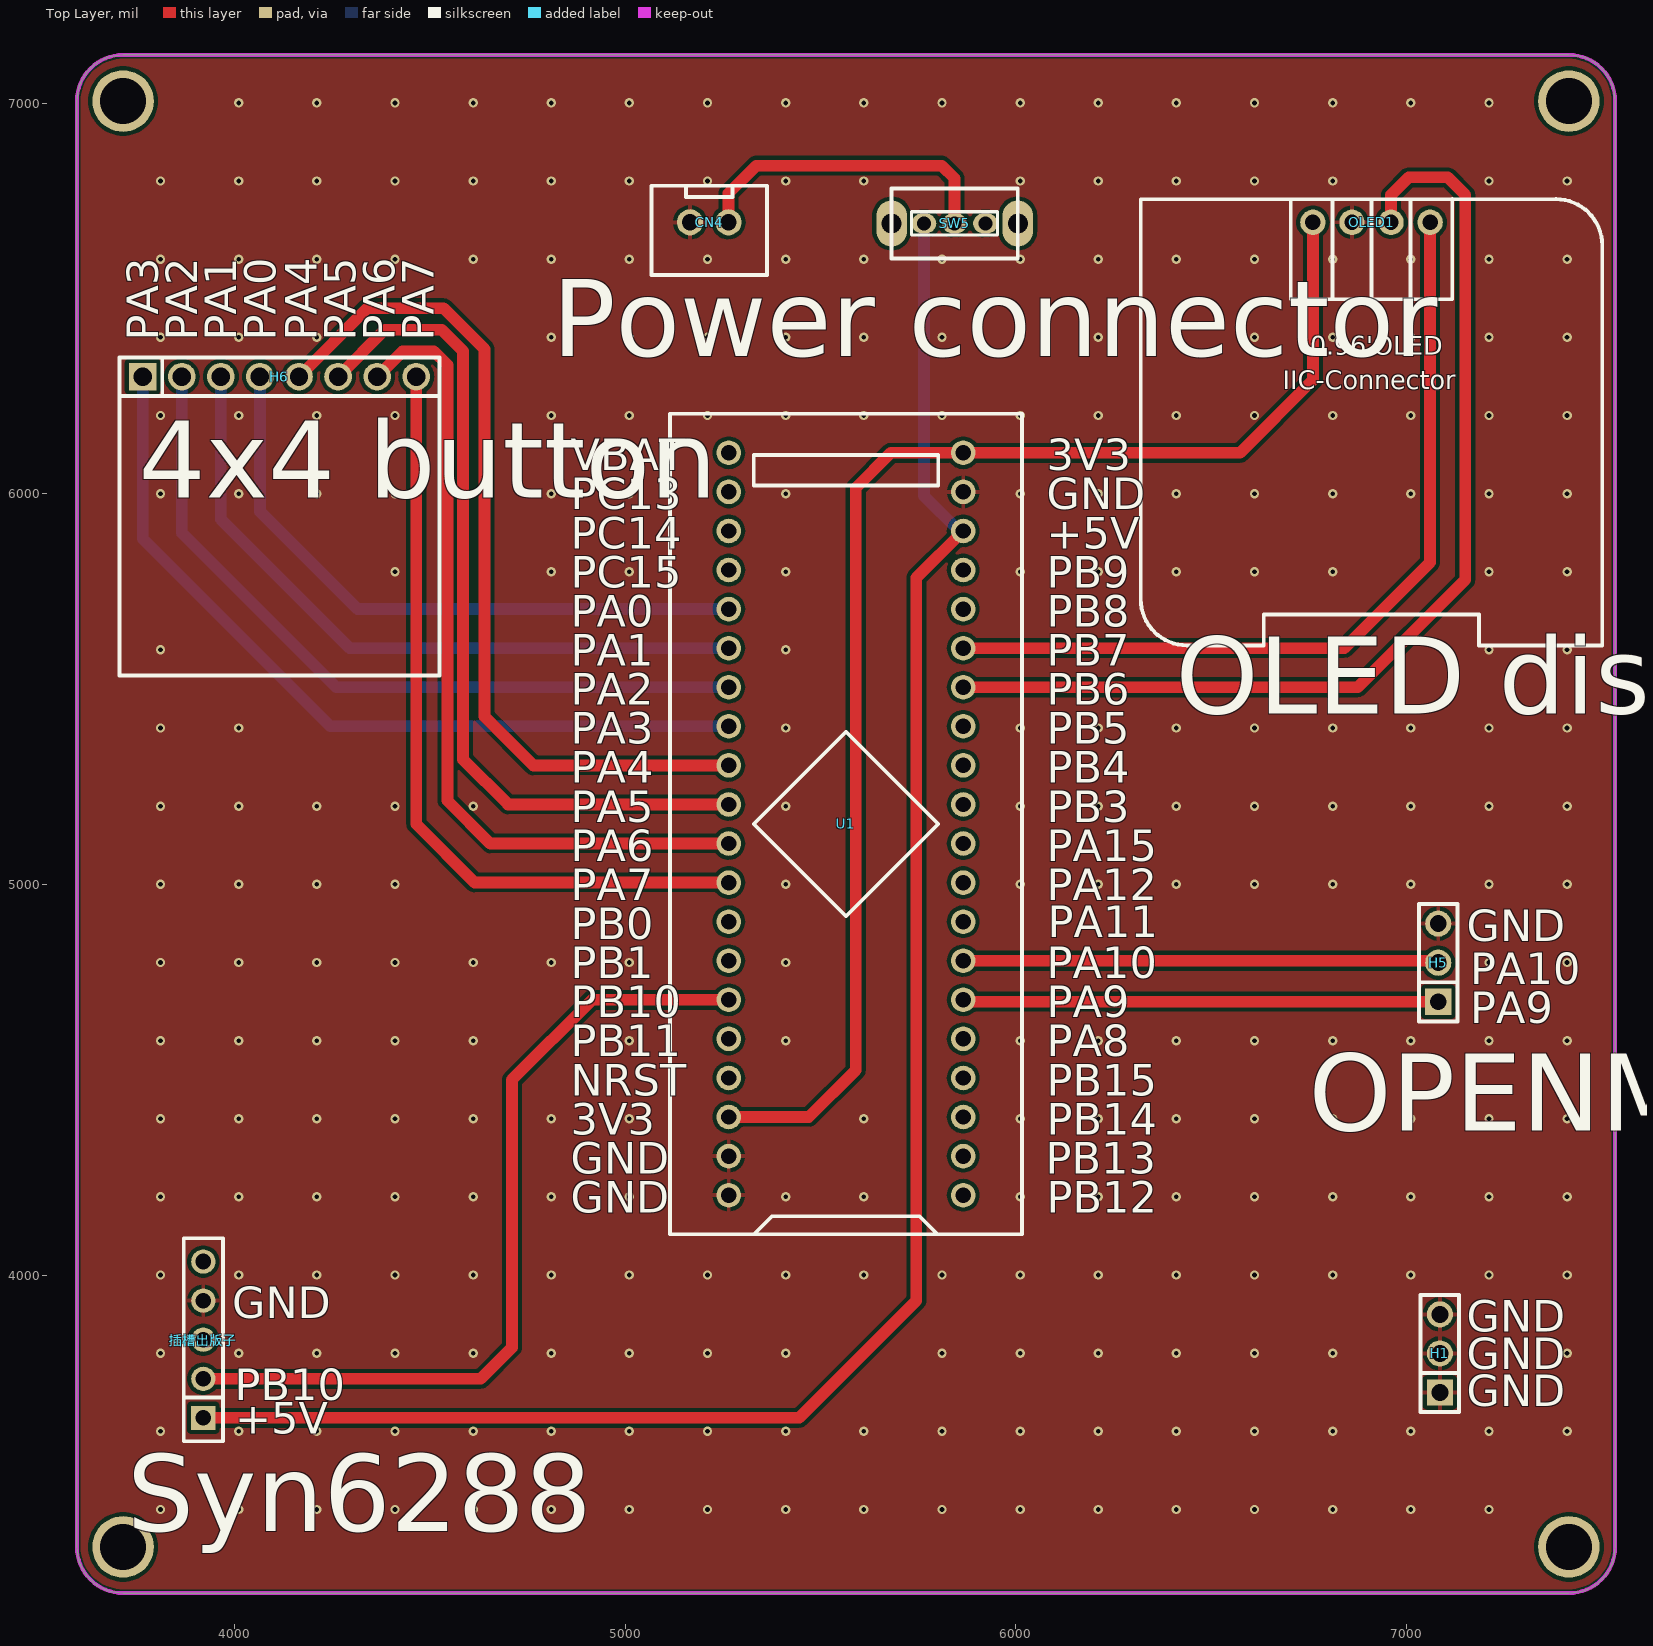
[diagram p0: Top Layer view]
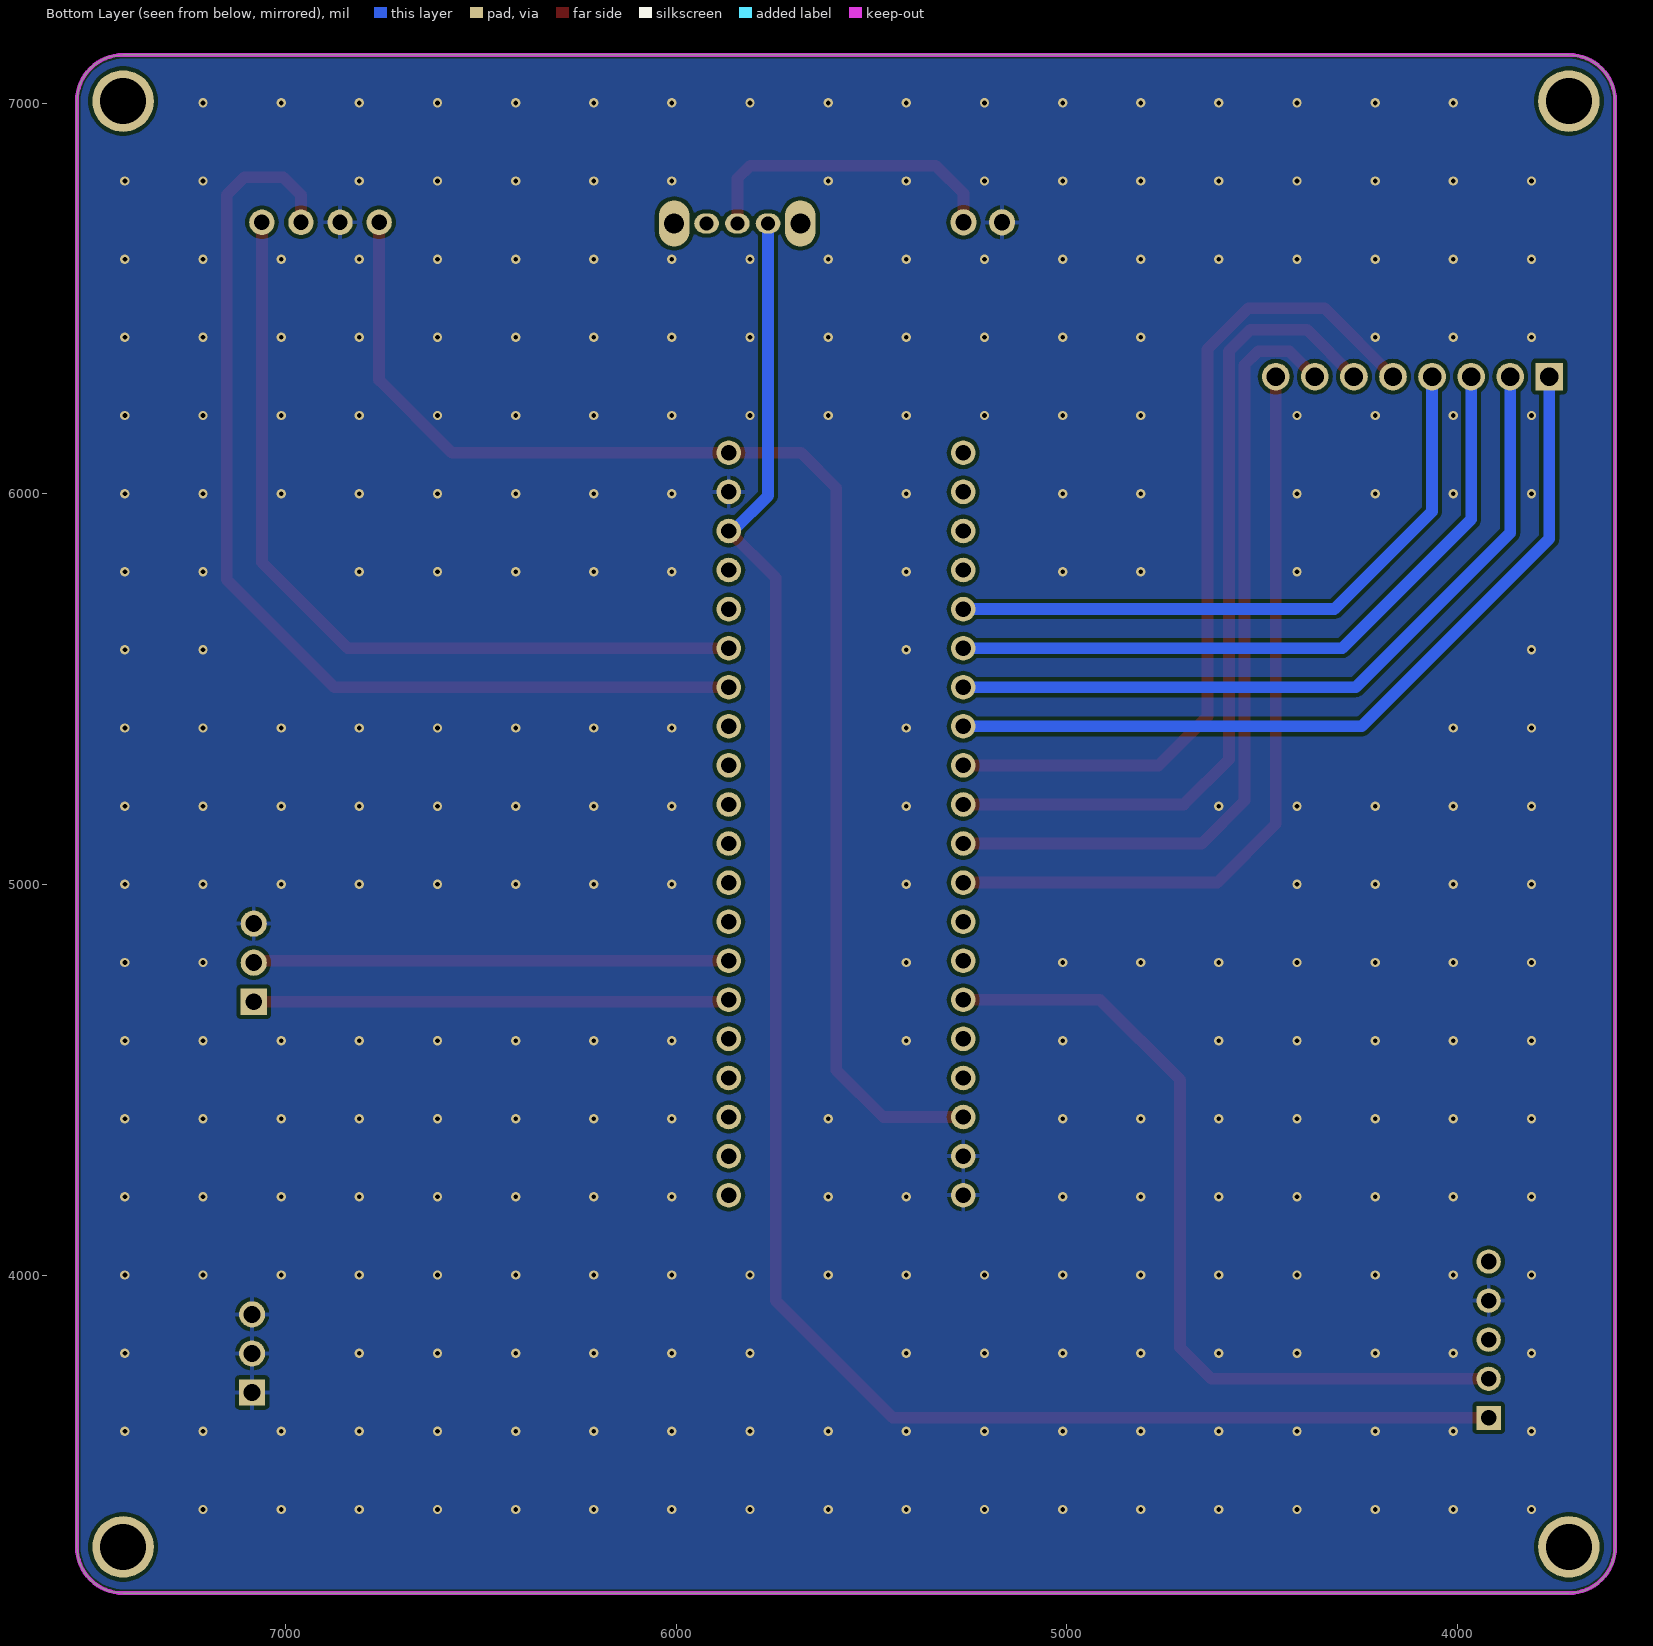
[diagram p1: Bottom Layer view, seen from below]
# Altium PCB MISC51713.pcbdoc
Units mil, origin at the board's own origin, x right, y up, seen from the top; angles counter-clockwise.
Board outline 3937.01 x 3937.01 mil, 2 copper layers (Top Layer, Bottom Layer), stack 62.206 mil thick; 8 components, 38 nets, 74 pads, 286 vias.

## Layer stack, top to bottom
Top Solder Mask Layer: solder mask 0.394, Dk 3.3
Top Layer: signal copper 1.379
Dielectric1: surface 59.449, FR4, Dk 4.5
Bottom Layer: signal copper 1.378
Bottom Solder Mask Layer: solder mask 0.394, Dk 3.3

## Board outline
3714.61,7123.5 ccw(c3714.61,7005.39) 3596.5,7005.39 3596.5,3304.61 ccw(c3714.61,3304.61) 3714.61,3186.5 7415.39,3186.5 ccw(c7415.39,3304.61) 7533.5,3304.61 7533.5,7005.39 ccw(c7415.39,7005.39) 7415.39,7123.5 3714.61,7123.5

## Design rules (kind name [scope] priority, off if disabled: settings)
BoardOutlineClearance copperThickness2oz_1 [All] p2 off: genericclearance=7.99 ignorepadtopadclearanceinfootprint=FALSE except(0: Arc-SplitContinuation Track-SplitContinuation SMDPad-SplitContinuation THPad-SplitContinuation Via-SplitContinuation Fill-SplitContinuation Region-SplitContinuation Poly-SplitContinuation Text-SplitContinuation Hole-SplitContinuation; 5.98: Arc-CutoutEdge Track-CutoutEdge SMDPad-CutoutEdge THPad-CutoutEdge Via-CutoutEdge Text-CutoutEdge; 6.9: Hole-OutlineEdge Hole-CutoutEdge; 10: Poly-OutlineEdge Poly-CutoutEdge; 11.81: Arc-OutlineEdge Track-OutlineEdge SMDPad-OutlineEdge THPad-OutlineEdge Via-OutlineEdge Fill-OutlineEdge Region-OutlineEdge Text-OutlineEdge Fill-CutoutEdge Region-CutoutEdge)
BoardOutlineClearance Plane_innerPlane_1 [All] p4 off: genericclearance=4.02 ignorepadtopadclearanceinfootprint=FALSE except(0: Arc-SplitContinuation Track-SplitContinuation SMDPad-SplitContinuation THPad-SplitContinuation Via-SplitContinuation Fill-SplitContinuation Region-SplitContinuation Poly-SplitContinuation Text-SplitContinuation Hole-SplitContinuation; 5.98: Arc-CutoutEdge Track-CutoutEdge SMDPad-CutoutEdge THPad-CutoutEdge Via-CutoutEdge Text-CutoutEdge; 6.9: Hole-OutlineEdge Hole-CutoutEdge; 10: Poly-OutlineEdge Poly-CutoutEdge; 11.81: Arc-OutlineEdge Track-OutlineEdge SMDPad-OutlineEdge THPad-OutlineEdge Via-OutlineEdge Fill-OutlineEdge Region-OutlineEdge Text-OutlineEdge Fill-CutoutEdge Region-CutoutEdge)
BoardOutlineClearance Copper_copperRegion_1 [All] p6 off: genericclearance=4.02 ignorepadtopadclearanceinfootprint=FALSE except(0: Arc-SplitContinuation Track-SplitContinuation SMDPad-SplitContinuation THPad-SplitContinuation Via-SplitContinuation Fill-SplitContinuation Region-SplitContinuation Poly-SplitContinuation Text-SplitContinuation Hole-SplitContinuation; 5.98: Arc-CutoutEdge Track-CutoutEdge SMDPad-CutoutEdge THPad-CutoutEdge Via-CutoutEdge Text-CutoutEdge; 6.9: Hole-OutlineEdge Hole-CutoutEdge; 10: Poly-OutlineEdge Poly-CutoutEdge; 11.81: Arc-OutlineEdge Track-OutlineEdge SMDPad-OutlineEdge THPad-OutlineEdge Via-OutlineEdge Fill-OutlineEdge Region-OutlineEdge Text-OutlineEdge Fill-CutoutEdge Region-CutoutEdge)
BoardOutlineClearance Copper_copperRegion_copperThickness1oz_1 [All] p8 off: genericclearance=4.02 ignorepadtopadclearanceinfootprint=FALSE except(0: Arc-SplitContinuation Track-SplitContinuation SMDPad-SplitContinuation THPad-SplitContinuation Via-SplitContinuation Fill-SplitContinuation Region-SplitContinuation Poly-SplitContinuation Text-SplitContinuation Hole-SplitContinuation; 5.98: Arc-CutoutEdge Track-CutoutEdge SMDPad-CutoutEdge THPad-CutoutEdge Via-CutoutEdge Text-CutoutEdge; 6.9: Hole-OutlineEdge Hole-CutoutEdge; 10: Poly-OutlineEdge Poly-CutoutEdge; 11.81: Arc-OutlineEdge Track-OutlineEdge SMDPad-OutlineEdge THPad-OutlineEdge Via-OutlineEdge Fill-OutlineEdge Region-OutlineEdge Text-OutlineEdge Fill-CutoutEdge Region-CutoutEdge)
BoardOutlineClearance Copper_copperRegion_Copper_copperRegion_1 [All] p10 off: genericclearance=4.02 ignorepadtopadclearanceinfootprint=FALSE except(0: Arc-SplitContinuation Track-SplitContinuation SMDPad-SplitContinuation THPad-SplitContinuation Via-SplitContinuation Fill-SplitContinuation Region-SplitContinuation Poly-SplitContinuation Text-SplitContinuation Hole-SplitContinuation; 5.98: Arc-CutoutEdge Track-CutoutEdge SMDPad-CutoutEdge THPad-CutoutEdge Via-CutoutEdge Text-CutoutEdge; 6.9: Hole-OutlineEdge Hole-CutoutEdge; 10: Poly-OutlineEdge Poly-CutoutEdge; 11.81: Arc-OutlineEdge Track-OutlineEdge SMDPad-OutlineEdge THPad-OutlineEdge Via-OutlineEdge Fill-OutlineEdge Region-OutlineEdge Text-OutlineEdge Fill-CutoutEdge Region-CutoutEdge)
BoardOutlineClearance copperThickness1oz_1 [All] p12: genericclearance=4.02 ignorepadtopadclearanceinfootprint=FALSE except(0: Arc-SplitContinuation Track-SplitContinuation SMDPad-SplitContinuation THPad-SplitContinuation Via-SplitContinuation Fill-SplitContinuation Region-SplitContinuation Poly-SplitContinuation Text-SplitContinuation Hole-SplitContinuation; 5.98: Arc-CutoutEdge Track-CutoutEdge SMDPad-CutoutEdge THPad-CutoutEdge Via-CutoutEdge Text-CutoutEdge; 6.9: Hole-OutlineEdge Hole-CutoutEdge; 10: Poly-OutlineEdge Poly-CutoutEdge; 11.81: Arc-OutlineEdge Track-OutlineEdge SMDPad-OutlineEdge THPad-OutlineEdge Via-OutlineEdge Fill-OutlineEdge Region-OutlineEdge Text-OutlineEdge Fill-CutoutEdge Region-CutoutEdge)
Clearance copperThickness2oz [All] p1 off: gap=7.99 ignorepadtopadclearanceinfootprint=FALSE except(5.98: SMDPad-Track SMDPad-SMDPad THPad-Track SMDPad-THPad THPad-THPad Track-Via SMDPad-Via THPad-Via Via-Via Fill-SMDPad Region-SMDPad Fill-THPad Region-THPad Fill-Via Region-Via Fill-Fill Fill-Region Region-Region Arc-Track Arc-SMDPad Arc-THPad Arc-Via Fill-Arc Region-Arc Arc-Arc Text-Track SMDPad-Text Text-THPad Text-Via Fill-Text Region-Text Arc-Text Text-Text; 6.9: Hole-Track Hole-SMDPad Hole-THPad Hole-Via Fill-Hole Region-Hole Hole-Arc Hole-Text; 10: Poly-Track Poly-SMDPad Poly-THPad Poly-Via Poly-Fill Poly-Region Poly-Poly Poly-Arc Poly-Text Poly-Hole; 11.81: Fill-Track Region-Track)
Clearance Plane_innerPlane [All] p3 off: gap=4.02 ignorepadtopadclearanceinfootprint=FALSE except(5.98: SMDPad-Track SMDPad-SMDPad THPad-Track SMDPad-THPad THPad-THPad Track-Via SMDPad-Via THPad-Via Via-Via Fill-SMDPad Region-SMDPad Fill-THPad Region-THPad Fill-Via Region-Via Fill-Fill Fill-Region Region-Region Arc-Track Arc-SMDPad Arc-THPad Arc-Via Fill-Arc Region-Arc Arc-Arc Text-Track SMDPad-Text Text-THPad Text-Via Fill-Text Region-Text Arc-Text Text-Text; 6.9: Hole-Track Hole-SMDPad Hole-THPad Hole-Via Fill-Hole Region-Hole Hole-Arc Hole-Text; 10: Poly-Track Poly-SMDPad Poly-THPad Poly-Via Poly-Fill Poly-Region Poly-Poly Poly-Arc Poly-Text Poly-Hole; 11.81: Fill-Track Region-Track)
Clearance Copper_copperRegion [All] p5 off: gap=4.02 ignorepadtopadclearanceinfootprint=FALSE except(5.98: SMDPad-Track SMDPad-SMDPad THPad-Track SMDPad-THPad THPad-THPad Track-Via SMDPad-Via THPad-Via Via-Via Fill-SMDPad Region-SMDPad Fill-THPad Region-THPad Fill-Via Region-Via Fill-Fill Fill-Region Region-Region Arc-Track Arc-SMDPad Arc-THPad Arc-Via Fill-Arc Region-Arc Arc-Arc Text-Track SMDPad-Text Text-THPad Text-Via Fill-Text Region-Text Arc-Text Text-Text; 6.9: Hole-Track Hole-SMDPad Hole-THPad Hole-Via Fill-Hole Region-Hole Hole-Arc Hole-Text; 10: Poly-Track Poly-SMDPad Poly-THPad Poly-Via Poly-Fill Poly-Region Poly-Poly Poly-Arc Poly-Text Poly-Hole; 11.81: Fill-Track Region-Track)
Clearance Copper_copperRegion_copperThickness1oz [All] p7 off: gap=4.02 ignorepadtopadclearanceinfootprint=FALSE except(5.98: SMDPad-Track SMDPad-SMDPad THPad-Track SMDPad-THPad THPad-THPad Track-Via SMDPad-Via THPad-Via Via-Via Fill-SMDPad Region-SMDPad Fill-THPad Region-THPad Fill-Via Region-Via Fill-Fill Fill-Region Region-Region Arc-Track Arc-SMDPad Arc-THPad Arc-Via Fill-Arc Region-Arc Arc-Arc Text-Track SMDPad-Text Text-THPad Text-Via Fill-Text Region-Text Arc-Text Text-Text; 6.9: Hole-Track Hole-SMDPad Hole-THPad Hole-Via Fill-Hole Region-Hole Hole-Arc Hole-Text; 10: Poly-Track Poly-SMDPad Poly-THPad Poly-Via Poly-Fill Poly-Region Poly-Poly Poly-Arc Poly-Text Poly-Hole; 11.81: Fill-Track Region-Track)
Clearance Copper_copperRegion_Copper_copperRegion [All] p9 off: gap=4.02 ignorepadtopadclearanceinfootprint=FALSE except(5.98: SMDPad-Track SMDPad-SMDPad THPad-Track SMDPad-THPad THPad-THPad Track-Via SMDPad-Via THPad-Via Via-Via Fill-SMDPad Region-SMDPad Fill-THPad Region-THPad Fill-Via Region-Via Fill-Fill Fill-Region Region-Region Arc-Track Arc-SMDPad Arc-THPad Arc-Via Fill-Arc Region-Arc Arc-Arc Text-Track SMDPad-Text Text-THPad Text-Via Fill-Text Region-Text Arc-Text Text-Text; 6.9: Hole-Track Hole-SMDPad Hole-THPad Hole-Via Fill-Hole Region-Hole Hole-Arc Hole-Text; 10: Poly-Track Poly-SMDPad Poly-THPad Poly-Via Poly-Fill Poly-Region Poly-Poly Poly-Arc Poly-Text Poly-Hole; 11.81: Fill-Track Region-Track)
Clearance copperThickness1oz [All] p11: gap=4.02 ignorepadtopadclearanceinfootprint=FALSE except(5.98: SMDPad-Track SMDPad-SMDPad THPad-Track SMDPad-THPad THPad-THPad Track-Via SMDPad-Via THPad-Via Via-Via Fill-SMDPad Region-SMDPad Fill-THPad Region-THPad Fill-Via Region-Via Fill-Fill Fill-Region Region-Region Arc-Track Arc-SMDPad Arc-THPad Arc-Via Fill-Arc Region-Arc Arc-Arc Text-Track SMDPad-Text Text-THPad Text-Via Fill-Text Region-Text Arc-Text Text-Text; 6.9: Hole-Track Hole-SMDPad Hole-THPad Hole-Via Fill-Hole Region-Hole Hole-Arc Hole-Text; 10: Poly-Track Poly-SMDPad Poly-THPad Poly-Via Poly-Fill Poly-Region Poly-Poly Poly-Arc Poly-Text Poly-Hole; 11.81: Fill-Track Region-Track)
DiffPairsRouting differentialPair [All] p1: maxlimit=6 minlimit=6 mostfreqgap=6 toplayer_minwidth=5 toplayer_prefwidth=10 toplayer_maxwidth=100 toplayer_mingap=6 toplayer_prefgap=6 toplayer_maxgap=6 bottomlayer_minwidth=5 bottomlayer_prefwidth=10 bottomlayer_maxwidth=100 bottomlayer_mingap=6 bottomlayer_prefgap=6 bottomlayer_maxgap=6 maxuncoupledlength=10
HoleToHoleClearance otherClearance [All] p1: gap=11.81 allowstackedmicrovias=TRUE
Length netLength [All] p1: minlimit=0 maxlimit=0
PasteMaskExpansion pasteMaskExpansion [All] p1: expansion=0
PlaneConnect innerPlane [All] p1: planeconnectstyle=Relief reliefexpansion=20 reliefentries=4 reliefconductorwidth=10 reliefairgap=10
PolygonConnect copperRegion_copperThickness1oz [All] p1 off: connectstyle=Relief reliefconductorwidth=10 reliefentries=4 polygonreliefangle="90 Angle" airgapwidth=10 via.connectstyle=Relief via.reliefconductorwidth=10 via.reliefentries=4 via.polygonreliefangle="90 Angle" via.airgapwidth=10
PolygonConnect copperRegion_Copper_copperRegion [All] p2 off: connectstyle=Relief reliefconductorwidth=10 reliefentries=4 polygonreliefangle="90 Angle" airgapwidth=10 via.connectstyle=Relief via.reliefconductorwidth=10 via.reliefentries=4 via.polygonreliefangle="90 Angle" via.airgapwidth=10
PolygonConnect copperRegion [All] p3: connectstyle=Relief reliefconductorwidth=10 reliefentries=4 polygonreliefangle="90 Angle" airgapwidth=10 via.connectstyle=Relief via.reliefconductorwidth=10 via.reliefentries=4 via.polygonreliefangle="90 Angle" via.airgapwidth=10
RoutingVias viaSize [All] p1: holewidth=12.01 width=24.02 viastyle="Through Hole" minholewidth=11.81 minwidth=19.68 maxholewidth=248.03 maxwidth=393.7
SolderMaskExpansion solderMaskExpansion [IsVia] p1: expansion=-1000 istentingtop=TRUE
SolderMaskExpansion solderMaskExpansion [All] p2: expansion=2 istentingtop=FALSE
Width copperThickness2oz_2 [All] p1 off: maxlimit=100 minlimit=8 preferedwidth=10
Width copperThickness1oz_2 [All] p2: maxlimit=100 minlimit=5 preferedwidth=10

## Components (designator, comment, footprint, x,y, rotation, side; value= is the part's Value field where it differs from the comment)
CN4 "XH2.54*2P_Through-hole" CONN-TH_2P-P2.50-XH2.54-2P 5215,6695 r0 top
H1 "" HDR-TH_3P-P2.54-V-M 7085,3800 r90 top
H5 "" HDR-TH_3P-P2.54-V-M 7080.79,4800 r90 top
H6 "" HDR-TH_8P-P2.54-V-F-1 4115,6300 r0 top
OLED1 "" 0.96OLED_4P 6910,6695 r0 top
SW5 "" 拨动开关 5837.9,6692.05 r0 top
U1 "STM32F103C8T6-Card" CONN-TH_L53.3-W22.9_STM32F103C8T6-CARD 5565,5155 r90 top
插槽出版子 "" HDR-TH_5P-P2.54-V-F 3920,3835 r90 top

## Footprints (in the part's own frame and the unit in brackets; to place one, negate y for a bottom-side part, rotate by r counter-clockwise, add the part's x,y. Pads: shape width x height; smd on the part's side, far side on the other; paste and mask are expansions set on the pad)
0.96OLED_4P [mm]
  round 1.65 hole 1 copper offset 0,0: 1(-3.81,-0.001) 2(-1.27,0.002) 3(1.27,0.002) 4(3.81,0.002)
  silkscreen extent -15,-27.5 15,1.5
CONN-TH_2P-P2.50-XH2.54-2P [mm]
  round 1.7 hole 1.05 paste+0 mask+0.05: 1(1.25,0) 2(-1.25,0)
  silkscreen extent -3.75,-3.42 3.75,2.37
CONN-TH_L53.3-W22.9_STM32F103C8T6-CARD [mm]
  round 1.6 hole 1: 1(-24.13,-7.62) 2(-21.59,-7.62) 3(-19.05,-7.62) 4(-16.51,-7.62) 5(-13.97,-7.62) 6(-11.43,-7.62) 7(-8.89,-7.62) 8(-6.35,-7.62) 9(-3.81,-7.62) 10(-1.27,-7.62) 11(1.27,-7.62) 12(3.81,-7.62) 13(6.35,-7.62) 14(8.89,-7.62) 15(11.43,-7.62) 16(13.97,-7.62) 17(16.51,-7.62) 18(19.05,-7.62) 19(21.59,-7.62) 20(24.13,-7.62) 21(24.13,7.62) 22(21.59,7.62) 23(19.05,7.62) 24(16.51,7.62) 25(13.97,7.62) 26(11.43,7.62) 27(8.89,7.62) 28(6.35,7.62) 29(3.81,7.62) 30(1.27,7.62) 31(-1.27,7.62) 32(-3.81,7.62) 33(-6.35,7.62) 34(-8.89,7.62) 35(-11.43,7.62) 36(-13.97,7.62) 37(-16.51,7.62) 38(-19.05,7.62) 39(-21.59,7.62) 40(-24.13,7.62)
  silkscreen extent -26.67,-11.43 26.67,11.43
HDR-TH_3P-P2.54-V-M [mm]
  rect 1.7x1.7 hole 1.1: 1(-2.54,0)
  round 1.7 hole 1.1: 2(0,0) 3(2.54,0)
  silkscreen extent -3.81,-1.25 3.81,1.25
HDR-TH_5P-P2.54-V-F [mil]
  rect 62x62 hole 40.16: 1(-200,0)
  round 62 hole 40.16: 2(-100,0) 3(0,0) 4(100,0) 5(200,0)
  silkscreen extent -260,-50 260,50
HDR-TH_8P-P2.54-V-F-1 [mm]
  rect 1.8x1.8 hole 1.2: 1(-8.89,0)
  round 1.8 hole 1.2: 2(-6.35,0) 3(-3.81,0) 4(-1.27,0) 5(1.27,0) 6(3.81,0) 7(6.35,0) 8(8.89,0)
  silkscreen extent -10.41,-1.25 10.41,1.25
拨动开关 [mil]
  oval 63x51.2 hole 35.4 paste+0 mask+2: 1(-73.4,0) 2(5,0) 3(84,0)
  oval 78.7x118.1 hole 51.2 paste+0 mask+2: 4(166.7,0) 5(-156.1,0)
  silkscreen extent -156,-90 167,90

## Free pads (board coordinates)
  round 157.48 hole 118.11: 1(3714.61,7005.39) 1(3714.61,3304.61) 1(7415.39,7005.39) 1(7415.39,3304.61)

## Via types
v1: diameter 24.02, hole 12, Top Layer to Bottom Layer, 286 vias

## Nets (pads, with @x,y where several pads share a name; then routed paths per layer and width w, separated by ;. In a path a pad name is that pad's centre, name@x,y a point inside that pad or via, vN(x,y) a via of type N, cw(c..) or ccw(c..) an arc to the next point about the centre after c; other vN are vias at no path point)
$1N17118: CN4.1 SW5.2 | length 810.9
  Top Layer w30: CN4.1 5264.22,6769.22 5335,6840 5810,6840 5842.9,6807.1 SW5.2
+5V: SW5.1 U1.18 插槽出版子.1 | length 4803.5
  Top Layer w30: 插槽出版子.1 5445,3635 5745,3935 5745,5785 U1.18
  Bottom Layer w30: SW5.1 5764.5,5995.5 5855,5905 U1.18
GND: CN4.2 H1.1 H1.2 H1.3 H5.3 OLED1.2 U1.19 U1.39 U1.40 插槽出版子.4
  other v1: 3810.6,3400.6 4010.6,3400.6 4210.6,3400.6 4410.6,3400.6 4610.6,3400.6 4810.6,3400.6 5010.6,3400.6 5210.6,3400.6 5410.6,3400.6 5610.6,3400.6 5810.6,3400.6 6010.6,3400.6 6210.6,3400.6 6410.6,3400.6 6610.6,3400.6 6810.6,3400.6 7010.6,3400.6 7210.6,3400.6 3810.6,3600.6 4010.6,3600.6 4210.6,3600.6 4410.6,3600.6 4610.6,3600.6 4810.6,3600.6 5010.6,3600.6 5210.6,3600.6 5410.6,3600.6 5610.6,3600.6 5810.6,3600.6 6010.6,3600.6 6210.6,3600.6 6410.6,3600.6 6610.6,3600.6 6810.6,3600.6 7010.6,3600.6 7210.6,3600.6 7410.6,3600.6 3810.6,3800.6 4010.6,3800.6 4210.6,3800.6 4410.6,3800.6 4610.6,3800.6 4810.6,3800.6 5010.6,3800.6 5210.6,3800.6 5410.6,3800.6 5810.6,3800.6 6010.6,3800.6 6210.6,3800.6 6410.6,3800.6 6610.6,3800.6 6810.6,3800.6 7410.6,3800.6 3810.6,4000.6 4010.6,4000.6 4210.6,4000.6 4410.6,4000.6 4610.6,4000.6 4810.6,4000.6 5010.6,4000.6 5210.6,4000.6 5410.6,4000.6 5610.6,4000.6 5810.6,4000.6 6010.6,4000.6 6210.6,4000.6 6410.6,4000.6 6610.6,4000.6 6810.6,4000.6 7010.6,4000.6 7210.6,4000.6 7410.6,4000.6 3810.6,4200.6 4010.6,4200.6 4210.6,4200.6 4410.6,4200.6 4610.6,4200.6 4810.6,4200.6 5010.6,4200.6 5410.6,4200.6 5610.6,4200.6 6010.6,4200.6 6210.6,4200.6 6410.6,4200.6 6610.6,4200.6 6810.6,4200.6 7010.6,4200.6 7210.6,4200.6 7410.6,4200.6 3810.6,4400.6 4010.6,4400.6 4210.6,4400.6 4410.6,4400.6 4610.6,4400.6 4810.6,4400.6 5010.6,4400.6 5610.6,4400.6 6010.6,4400.6 6210.6,4400.6 6410.6,4400.6 6610.6,4400.6 6810.6,4400.6 7010.6,4400.6 7210.6,4400.6 7410.6,4400.6 3810.6,4600.6 4010.6,4600.6 4210.6,4600.6 4410.6,4600.6 4610.6,4600.6 5010.6,4600.6 5410.6,4600.6 6010.6,4600.6 6210.6,4600.6 6410.6,4600.6 6610.6,4600.6 6810.6,4600.6 7010.6,4600.6 7210.6,4600.6 7410.6,4600.6 3810.6,4800.6 4010.6,4800.6 4210.6,4800.6 4410.6,4800.6 4610.6,4800.6 4810.6,4800.6 5010.6,4800.6 5410.6,4800.6 7210.6,4800.6 7410.6,4800.6 3810.6,5000.6 4010.6,5000.6 4210.6,5000.6 4410.6,5000.6 5410.6,5000.6 6010.6,5000.6 6210.6,5000.6 6410.6,5000.6 6610.6,5000.6 6810.6,5000.6 7010.6,5000.6 7210.6,5000.6 7410.6,5000.6 3810.6,5200.6 4010.6,5200.6 4210.6,5200.6 4410.6,5200.6 4610.6,5200.6 5410.6,5200.6 6010.6,5200.6 6210.6,5200.6 6410.6,5200.6 6610.6,5200.6 6810.6,5200.6 7010.6,5200.6 7210.6,5200.6 7410.6,5200.6 3810.6,5400.6 4010.6,5400.6 5410.6,5400.6 6010.6,5400.6 6210.6,5400.6 6410.6,5400.6 6610.6,5400.6 6810.6,5400.6 7010.6,5400.6 7210.6,5400.6 7410.6,5400.6 3810.6,5600.6 5410.6,5600.6 7210.6,5600.6 7410.6,5600.6 4410.6,5800.6 4810.6,5800.6 5010.6,5800.6 5410.6,5800.6 6010.6,5800.6 6210.6,5800.6 6410.6,5800.6 6610.6,5800.6 6810.6,5800.6 7210.6,5800.6 7410.6,5800.6 3810.6,6000.6 4010.6,6000.6 4210.6,6000.6 4410.6,6000.6 4810.6,6000.6 5010.6,6000.6 5410.6,6000.6 6010.6,6000.6 6210.6,6000.6 6410.6,6000.6 6610.6,6000.6 6810.6,6000.6 7010.6,6000.6 7210.6,6000.6 7410.6,6000.6 3810.6,6200.6 4010.6,6200.6 4210.6,6200.6 4410.6,6200.6 4810.6,6200.6 5010.6,6200.6 5210.6,6200.6 5410.6,6200.6 5610.6,6200.6 5810.6,6200.6 6010.6,6200.6 6210.6,6200.6 6410.6,6200.6 6610.6,6200.6 6810.6,6200.6 7010.6,6200.6 7210.6,6200.6 7410.6,6200.6 3810.6,6400.6 4010.6,6400.6 4210.6,6400.6 4810.6,6400.6 5010.6,6400.6 5210.6,6400.6 5410.6,6400.6 5610.6,6400.6 5810.6,6400.6 6010.6,6400.6 6210.6,6400.6 6410.6,6400.6 6610.6,6400.6 6810.6,6400.6 7010.6,6400.6 7210.6,6400.6 7410.6,6400.6 3810.6,6600.6 4010.6,6600.6 4210.6,6600.6 4410.6,6600.6 4610.6,6600.6 4810.6,6600.6 5010.6,6600.6 5210.6,6600.6 5410.6,6600.6 5610.6,6600.6 5810.6,6600.6 6010.6,6600.6 6210.6,6600.6 6410.6,6600.6 6610.6,6600.6 6810.6,6600.6 7010.6,6600.6 7210.6,6600.6 7410.6,6600.6 3810.6,6800.6 4010.6,6800.6 4210.6,6800.6 4410.6,6800.6 4610.6,6800.6 4810.6,6800.6 5010.6,6800.6 5210.6,6800.6 5410.6,6800.6 5610.6,6800.6 6010.6,6800.6 6210.6,6800.6 6410.6,6800.6 6610.6,6800.6 6810.6,6800.6 7210.6,6800.6 7410.6,6800.6 4010.6,7000.6 4210.6,7000.6 4410.6,7000.6 4610.6,7000.6 4810.6,7000.6 5010.6,7000.6 5210.6,7000.6 5410.6,7000.6 5610.6,7000.6 5810.6,7000.6 6010.6,7000.6 6210.6,7000.6 6410.6,7000.6 6610.6,7000.6 6810.6,7000.6 7010.6,7000.6 7210.6,7000.6
NRST: U1.37
PA0: H6.4 U1.25 | length 1648.6
  Bottom Layer w30: H6.4 4065,5955 4315,5705 U1.25
PA1: H6.3 U1.26 | length 1801.7
  Bottom Layer w30: H6.3 3965,5935 4295,5605 U1.26
PA2: H6.2 U1.27 | length 1963.6
  Bottom Layer w30: H6.2 3865,5900 4260,5505 U1.27
PA3: H6.1 U1.28 | length 2113.8
  Bottom Layer w30: H6.1 3765,5885 4245,5405 U1.28
PA4: H6.5 U1.29 | length 2207.8
  Top Layer w30: H6.5 4340,6475 4535,6475 4640,6370 4640,5430 4765,5305 U1.29
PA5: H6.6 U1.30 | length 2165.1
  Top Layer w30: H6.6 4385,6420 4530,6420 4585,6365 4585,5320 4700,5205 U1.30
PA6: H6.7 U1.31 | length 2102
  Top Layer w30: H6.7 4430,6365 4510,6365 4545,6330 4545,5215 4655,5105 U1.31
PA7: H6.8 U1.32 | length 2007.1
  Top Layer w30: H6.8 4465,5155 4615,5005 U1.32
PA8: U1.5
PA9: H5.1 U1.6 | length 1217.9
  Top Layer w30: U1.6 5870,4700 H5.1
PA10: H5.2 U1.7 | length 1217.9
  Top Layer w30: U1.7 7075.79,4805 H5.2
PA11: U1.8
PA12: U1.9
PA15: U1.10
PB0: U1.33
PB1: U1.34
PB3: U1.11
PB4: U1.12
PB5: U1.13
PB6: OLED1.3 U1.14 | length 2681.1
  Top Layer w30: U1.14 6875,5505 7150,5780 7150,6765 7105,6810 7005,6810 6960,6765 OLED1.3@6960,6695.05
PB7: OLED1.4 U1.15 | length 2156.2
  Top Layer w30: U1.15 6840,5605 7060,5825 OLED1.4@7060,6695.05
PB8: U1.16
PB9: U1.17
PB10: U1.35 插槽出版子.2 | length 2148.1
  Top Layer w30: 插槽出版子.2 4630,3735 4710,3815 4710,4500 4915,4705 U1.35
PB11: U1.36
PB12: U1.1
PB13: U1.2
PB14: U1.3
PB15: U1.4
PC13: U1.22
PC14: U1.23
PC15: U1.24
VBAT: U1.21
VCC: OLED1.1 U1.20 U1.38 | length 3552.7
  Top Layer w30: U1.38 5470,4405 5590,4525 5590,6015 5680,6105 U1.20 6573.61,6105 6760,6291.4 OLED1.1
pads on no net: SW5.3 SW5.4 SW5.5 插槽出版子.3 插槽出版子.5

## Polygon pours and split planes (outlines as drawn)
GND on Bottom Layer (solid, remove dead copper, pour order 2): 3525,7245 3525,3080 7700,3080 7700,7245
GND on Top Layer (solid, remove dead copper, pour order 2): 3000,7415 3000,3000 7930,3000 7930,7415

## Keep-outs
Board Outline Layer:
  the board outline again, w10

## Silkscreen, mask and mechanical layers (free items; w line width, h text height)
Top Silkscreen Layer:
  lines w10: 3705.16,5535 3705.16,6349.21 4525,6349.21 4525,5535 3705.16,5535
  text "PA3" at 3805,6391.55 h80 r90
  text "PA2" at 3905,6391.55 h80 r90
  text "PA1" at 4005,6391.55 h80 r90
  text "PA0" at 4105,6391.55 h80 r90
  text "PA4" at 4210,6391.55 h80 r90
  text "PA5" at 4310,6391.55 h80 r90
  text "PA6" at 4410,6391.55 h80 r90
  text "PA7" at 4510,6391.55 h80 r90
  text "Power connector" at 4812.87,6351.57 h196.85
  text "VBAT" at 4860.95,6060 h80
  text "3V3" at 6079.16,6060 h80
  text "4x4 button" at 3755,5990 h196.85
  text "PC13" at 4860.95,5960 h80
  text "GND" at 6079.16,5960 h80
  text "PC14" at 4860.95,5860 h80
  text "+5V" at 6079.16,5860 h80
  text "PC15" at 4860.95,5760 h80
  text "PB9" at 6079.16,5760 h80
  text "PA0" at 4860.95,5660 h80
  text "PB8" at 6079.16,5660 h80
  text "PA1" at 4860.95,5560 h80
  text "PB7" at 6079.16,5560 h80
  text "PA2" at 4860.95,5460 h80
  text "PB6" at 6079.16,5460 h80
  text "OLED display" at 6408.66,5436.57 h196.85
  text "PA3" at 4860.95,5360 h80
  text "PB5" at 6079.16,5360 h80
  text "PA4" at 4860.95,5260 h80
  text "PB4" at 6079.16,5260 h80
  text "PA5" at 4860.95,5160 h80
  text "PB3" at 6079.16,5160 h80
  text "PA6" at 4860.95,5060 h80
  text "PA15" at 6079.16,5060 h80
  text "PA7" at 4860.95,4960 h80
  text "PA12" at 6079.16,4960 h80
  text "PA11" at 6080.95,4865 h80
  text "PB0" at 4860.95,4860 h80
  text "GND" at 7153.8,4855 h80
  text "PB1" at 4860.95,4760 h80
  text "PA10" at 6079.16,4760 h80
  text "PA10" at 7162.65,4745 h80
  text "PB10" at 4860.95,4660 h80
  text "PA9" at 6079.16,4660 h80
  text "PA9" at 7162.65,4645 h80
  text "PB11" at 4860.95,4560 h80
  text "PA8" at 6079.16,4560 h80
  text "NRST" at 4860.95,4460 h80
  text "PB15" at 6079.16,4460 h80
  text "OPENMV" at 6750,4370 h196.85
  text "3V3" at 4860.95,4360 h80
  text "PB14" at 6079.16,4360 h80
  text "GND" at 4860.95,4260 h80
  text "PB13" at 6075.95,4260 h80
  text "GND" at 4860.95,4160 h80
  text "PB12" at 6079.16,4160 h80
  text "GND" at 3993.8,3890 h80
  text "GND" at 7153.8,3855 h80
  text "GND" at 7153.8,3760 h80
  text "PB10" at 3999.9,3680 h80
  text "GND" at 7153.8,3665 h80
  text "+5V" at 4002.35,3595 h80
  text "Syn6288" at 3725,3345 h196.85